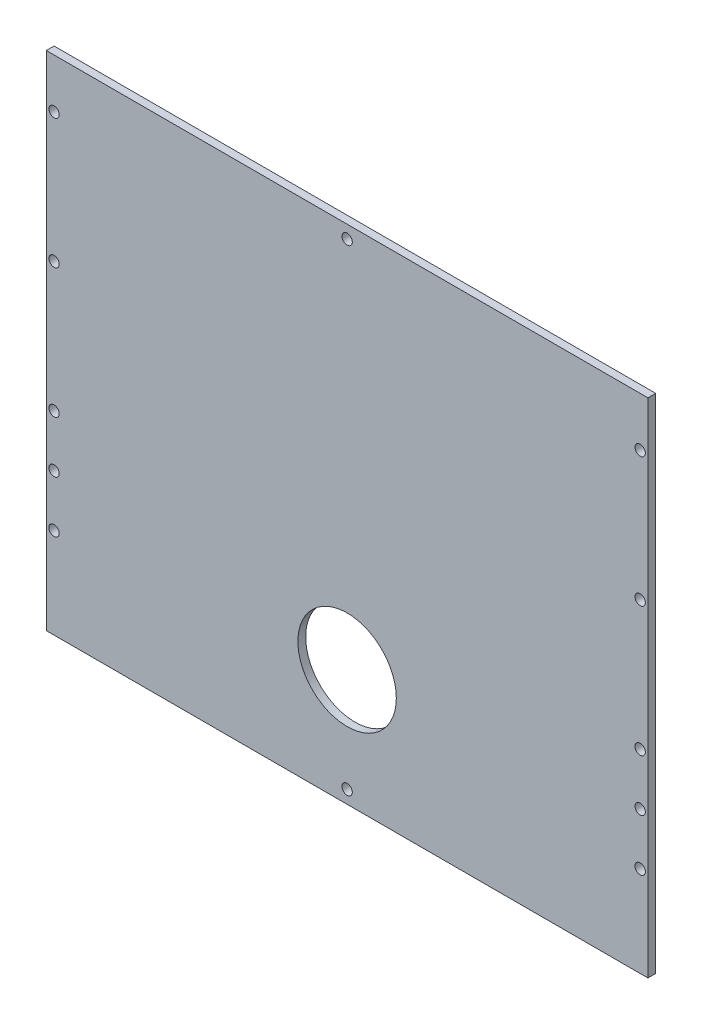
SolidWorks part; units mm, degrees
ref_plane "Front Plane" through (0, 0, 0) normal (0, 0, 1) x (1, 0, 0)
ref_plane "Top Plane" through (0, 0, 0) normal (0, 1, 0) x (1, 0, 0)
ref_plane "Right Plane" through (0, 0, 0) normal (1, 0, 0) x (0, 0, -1)
sketch "Sketch1" plane through (0, 0, 0) normal (0, 0, 1) x (1, 0, 0)
  line L1 (-116.15, 97) -> (116.15, 97)
  line L2 (-116.15, 97) -> (-116.15, -97)
  line L3 (-116.15, -97) -> (116.15, -97)
  line L4 (116.15, 97) -> (116.15, -97)
  line L5 (-116.15, 97) -> (116.15, -97) construction
  line L6 (-116.15, -97) -> (116.15, 97) construction
  point P0 (0, 0)
  dimension "D1" = 232.3
  dimension "D2" = 194
extrude "Boss-Extrude1" add sketch "Sketch1" along normal blind 3
sketch "Sketch2" plane through (0, 0, 3) normal (0, 0, 1) x (1, 0, 0)
  line L0 (-116.15, -97) -> (116.15, -97) construction
  circle A0 centre (0, -52) radius 19
  dimension "D1" = 38
  dimension "D2" = 45
extrude "Cut-Extrude1" cut sketch "Sketch2" against normal blind 3
sketch "Sketch3" plane through (0, 0, 3) normal (0, 0, 1) x (1, 0, 0)
  line L0 (-179.4196, 0) -> (165.8029, 0) construction
  line L1 (116.15, 97) -> (-116.15, 97) construction
  circle A0 centre (0, 92) radius 2
  circle A1 centre (0, -92) radius 2
  dimension "D1" = 4
  dimension "D2" = 5
extrude "Cut-Extrude2" cut sketch "Sketch3" against normal blind 4
sketch "Sketch4" plane through (0, 0, 3) normal (0, 0, 1) x (1, 0, 0)
  line L0 (-116.15, 97) -> (-116.15, -97) construction
  line L1 (-116.15, -97) -> (116.15, -97) construction
  circle A0 centre (-113.15, 78) radius 2
  circle A1 centre (-113.15, 28) radius 2
  circle A2 centre (-113.15, -22) radius 2
  circle A3 centre (-113.15, -42) radius 2
  circle A4 centre (-113.15, -62) radius 2
  dimension "D1" = 4
  dimension "D2" = 4
  dimension "D3" = 4
  dimension "D4" = 4
  dimension "D5" = 4
  dimension "D6" = 3
  dimension "D7" = 35
  dimension "D8" = 20
  dimension "D9" = 20
  dimension "D10" = 50
  dimension "D11" = 50
extrude "Cut-Extrude3" cut sketch "Sketch4" against normal through all
mirror "Mirror1" about plane through (0, 0, 0) normal (1, 0, 0) of "Cut-Extrude3"
